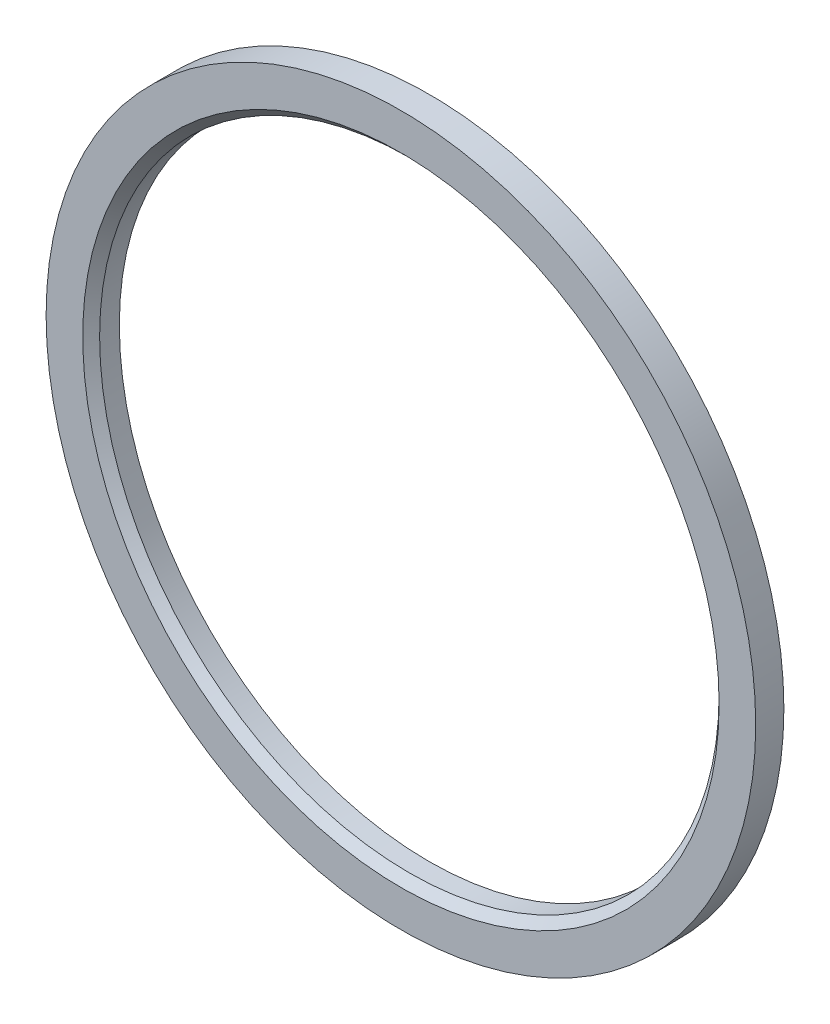
SolidWorks part; units mm, degrees
material "42CrMo"
ref_plane "Front Plane" through (0, 0, 0) normal (0, 0, 1) x (1, 0, 0)
ref_plane "Top Plane" through (0, 0, 0) normal (0, 1, 0) x (1, 0, 0)
ref_plane "Right Plane" through (0, 0, 0) normal (1, 0, 0) x (0, 0, -1)
sketch "Sketch1" plane through (0, 0, 0) normal (0, 0, 1) x (1, 0, 0)
  circle A0 centre (0, 0) radius 126
  circle A1 centre (0, 0) radius 110
  dimension "D1" = 252
  dimension "D2" = 220
extrude "Boss-Extrude1" add sketch "Sketch1" along normal blind 10
chamfer "Chamfer1" distance 3 angle 45 1 edges at (110, 0, 10)
